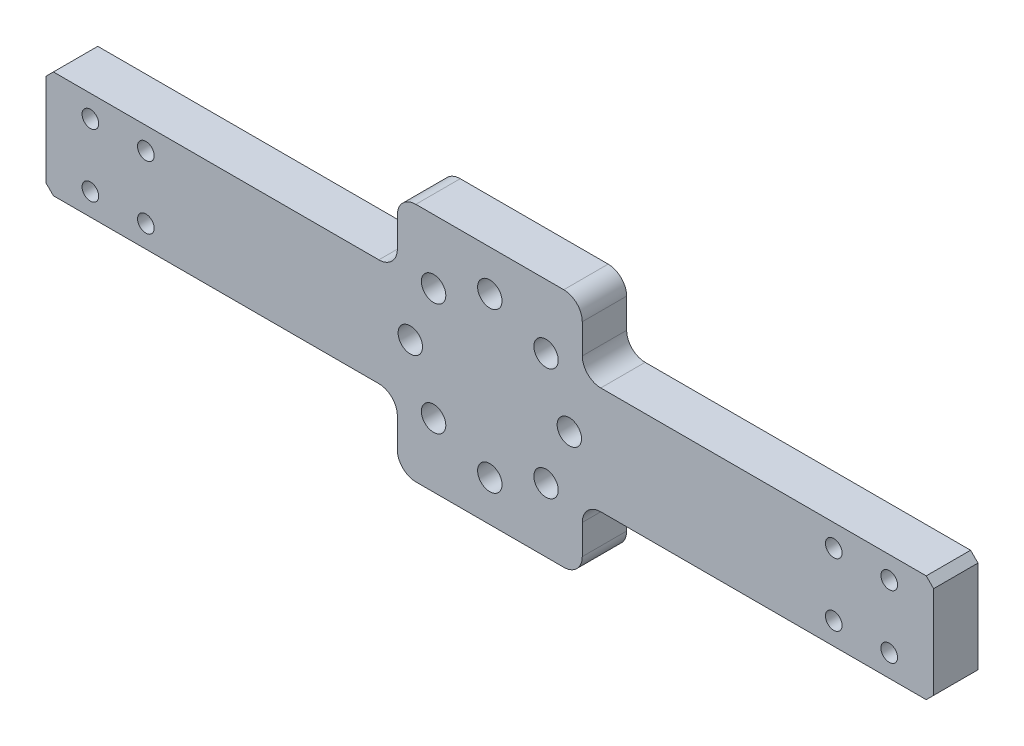
from build123d import *

# Parameters (mm, degrees)
SKETCH1_W                                        = 240
SKETCH1_H                                        = 65
BOSS_EXTRUDE1_DEPTH                              = 12
CUT_EXTRUDE1_DEPTH                               = 125.900960765
CUT_EXTRUDE1_DEPTH_BACK                          = 125.900960765
SKETCH2_W                                        = 95
SKETCH2_H                                        = 18
FILLET1_R                                        = 5
HOLE_FOR_SOCKET_HEAD_CAP_SCREW_TYPE1_D           = 6.6
HOLE_FOR_SOCKET_HEAD_CAP_SCREW_TYPE1_CBORE_D     = 11
HOLE_FOR_SOCKET_HEAD_CAP_SCREW_TYPE1_CBORE_DEPTH = 6.8
F_4_5_4_5_DIAMETER_HOLE1_D                       = 4.5
CHAMFER1_SIZE                                    = 2


with BuildPart() as part:
    # Sketch1 → Boss-Extrude1 (new body)
    with BuildSketch(Plane.XY):
        Rectangle(SKETCH1_W, SKETCH1_H)
    extrude(amount=BOSS_EXTRUDE1_DEPTH)

    # Sketch2 → Cut-Extrude1 (cut, two sides: drawn at the far end of the back side and taken through both)
    with BuildSketch(Plane.XY.offset(12).offset(-CUT_EXTRUDE1_DEPTH_BACK)):
        with Locations((-72.5, 23.5)):
            Rectangle(SKETCH2_W, SKETCH2_H)
        with Locations((72.5, 23.5)):
            Rectangle(SKETCH2_W, SKETCH2_H)
        with Locations((72.5, -23.5)):
            Rectangle(SKETCH2_W, SKETCH2_H)
        with Locations((-72.5, -23.5)):
            Rectangle(SKETCH2_W, SKETCH2_H)
    extrude(amount=CUT_EXTRUDE1_DEPTH + CUT_EXTRUDE1_DEPTH_BACK, mode=Mode.SUBTRACT)

    # Fillet1
    fillet1_edges = [part.edges().sort_by_distance(p)[0] for p in [
        (-25, -32.5, 6),
        (-25, -14.5, 6),
        (25, -32.5, 6),
        (25, -14.5, 6),
        (25, 32.5, 6),
        (25, 14.5, 6),
        (-25, 32.5, 6),
        (-25, 14.5, 6),
    ]]
    fillet(fillet1_edges, radius=FILLET1_R)

    # Hole for socket head cap screw, type1 (through all)
    with Locations(Plane(origin=(0, 0, 0), x_dir=(-1, 0, 0), z_dir=(0, 0, -1))):
        with Locations((15.202795796, -15.202795796), (0, -21.5), (-15.202795796, -15.202795796), (-21.5, 0), (-15.202795796, 15.202795796), (0, 21.5), (15.202795796, 15.202795796), (21.5, 0)):
            CounterBoreHole(HOLE_FOR_SOCKET_HEAD_CAP_SCREW_TYPE1_D / 2, HOLE_FOR_SOCKET_HEAD_CAP_SCREW_TYPE1_CBORE_D / 2, HOLE_FOR_SOCKET_HEAD_CAP_SCREW_TYPE1_CBORE_DEPTH)

    # Ø4.5 (4.5) Diameter Hole1 (through all)
    with Locations(Plane.XY.offset(12)):
        with Locations((-93, -8.5), (-108, -8.5), (-93, 8.5), (-108, 8.5)):
            f_4_5_4_5_diameter_hole1 = Hole(F_4_5_4_5_DIAMETER_HOLE1_D / 2)

    # Mirror1: Ø4.5 (4.5) Diameter Hole1 across plane
    add(f_4_5_4_5_diameter_hole1.mirror(Plane(origin=(0, 0, 0), x_dir=(0, 0, 1), z_dir=(1, 0, 0))), mode=Mode.SUBTRACT)

    # Chamfer1
    chamfer1_edges = [part.edges().sort_by_distance(p)[0] for p in [
        (-120, -14.5, 6),
        (120, -14.5, 6),
        (120, 14.5, 6),
        (-120, 14.5, 6),
    ]]
    chamfer(chamfer1_edges, length=CHAMFER1_SIZE)


solid = part.part
